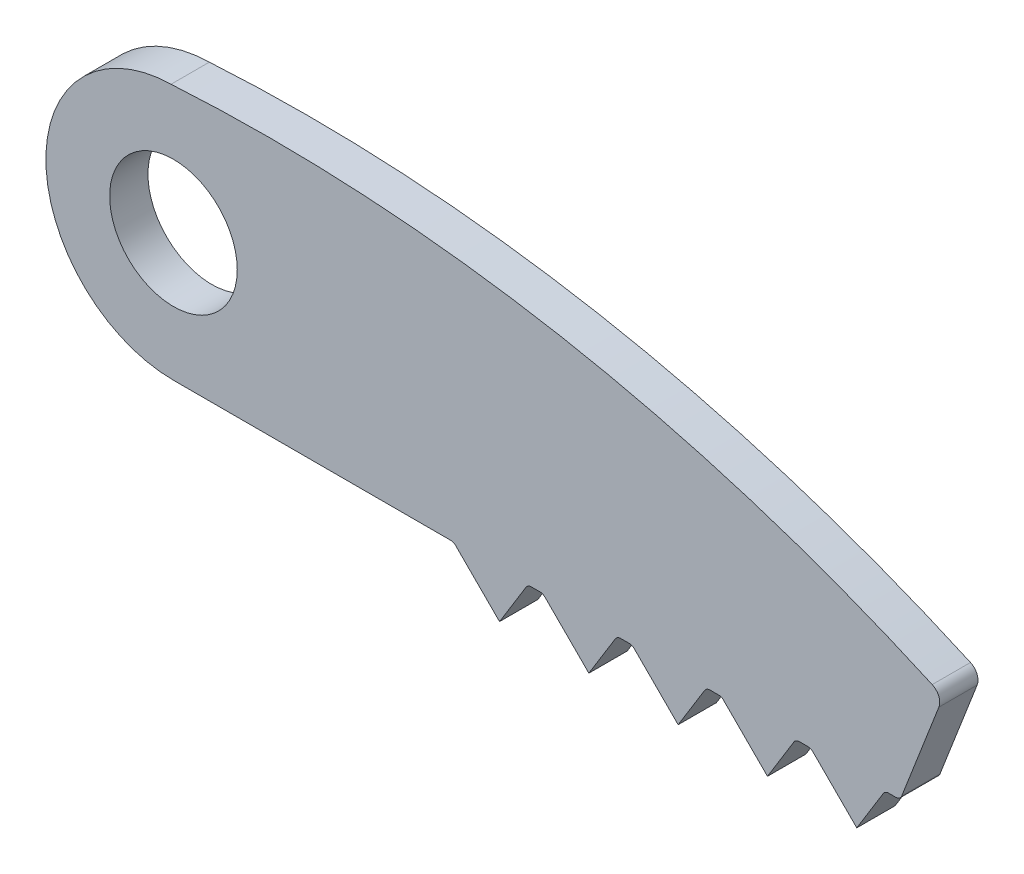
SolidWorks part; units mm, degrees
ref_plane "Front Plane" through (0, 0, 0) normal (0, 0, 1) x (1, 0, 0)
ref_plane "Top Plane" through (0, 0, 0) normal (0, 1, 0) x (1, 0, 0)
ref_plane "Right Plane" through (0, 0, 0) normal (1, 0, 0) x (0, 0, -1)
sketch "Sketch3" plane through (0, 0, 0) normal (0, 0, 1) x (1, 0, 0)
  line L0 (0, -10) -> (21.7479, -10)
  line L1 (22.1014, -10.1464) -> (25.5586, -13.6036)
  line L2 (25.5586, -13.6036) -> (27.6306, -10.2379)
  line L3 (28.0564, -10) -> (28.7479, -10)
  line L4 (35.0564, -10) -> (35.7479, -10)
  line L5 (32.5586, -13.6036) -> (34.6306, -10.2379)
  line L6 (29.1014, -10.1464) -> (32.5586, -13.6036)
  line L7 (42.0564, -10) -> (42.7479, -10)
  line L8 (39.5586, -13.6036) -> (41.6306, -10.2379)
  line L9 (36.1014, -10.1464) -> (39.5586, -13.6036)
  line L10 (49.0564, -10) -> (49.7479, -10)
  line L11 (46.5586, -13.6036) -> (48.6306, -10.2379)
  line L12 (43.1014, -10.1464) -> (46.5586, -13.6036)
  line L13 (56.0564, -10) -> (56.613, -10)
  line L14 (53.5586, -13.6036) -> (55.6306, -10.2379)
  line L15 (50.1014, -10.1464) -> (53.5586, -13.6036)
  line L17 (57.079, -9.6813) -> (59.9913, -2.1961)
  arc A0 (-0.189, 9.9982) -> (0, -10) centre (0, 0) ccw
  arc A3 (-0.189, 9.9982) -> (59.4702, -0.9218) centre (7.553, -116.1329) cw
  arc A4 (59.9913, -2.1961) -> (59.4702, -0.9218) centre (59.0593, -1.8335) ccw
  arc A5 (56.613, -10) -> (57.079, -9.6813) centre (56.613, -9.5) ccw
  arc A6 (55.6306, -10.2379) -> (56.0564, -10) centre (56.0564, -10.5) cw
  arc A7 (49.7479, -10) -> (50.1014, -10.1464) centre (49.7479, -10.5) cw
  arc A8 (49.0564, -10) -> (48.6306, -10.2379) centre (49.0564, -10.5) ccw
  arc A9 (42.7479, -10) -> (43.1014, -10.1464) centre (42.7479, -10.5) cw
  arc A10 (42.0564, -10) -> (41.6306, -10.2379) centre (42.0564, -10.5) ccw
  arc A11 (35.7479, -10) -> (36.1014, -10.1464) centre (35.7479, -10.5) cw
  arc A12 (35.0564, -10) -> (34.6306, -10.2379) centre (35.0564, -10.5) ccw
  arc A13 (28.7479, -10) -> (29.1014, -10.1464) centre (28.7479, -10.5) cw
  arc A14 (28.0564, -10) -> (27.6306, -10.2379) centre (28.0564, -10.5) ccw
  arc A15 (22.1014, -10.1464) -> (21.7479, -10) centre (21.7479, -10.5) ccw
  dimension "D1" = 20
  dimension "D2" = 1
  dimension "D4" = 0.5
  dimension "D5" = 0.5
  dimension "D3" = 5
extrude "Boss-Extrude3" add sketch "Sketch3" along normal blind 3
sketch "Sketch4" plane through (0, 0, 3) normal (0, 0, 1) x (1, 0, 0)
  circle A0 centre (0, 0) radius 5
extrude "Cut-Extrude1" cut sketch "Sketch4" against normal blind 3
